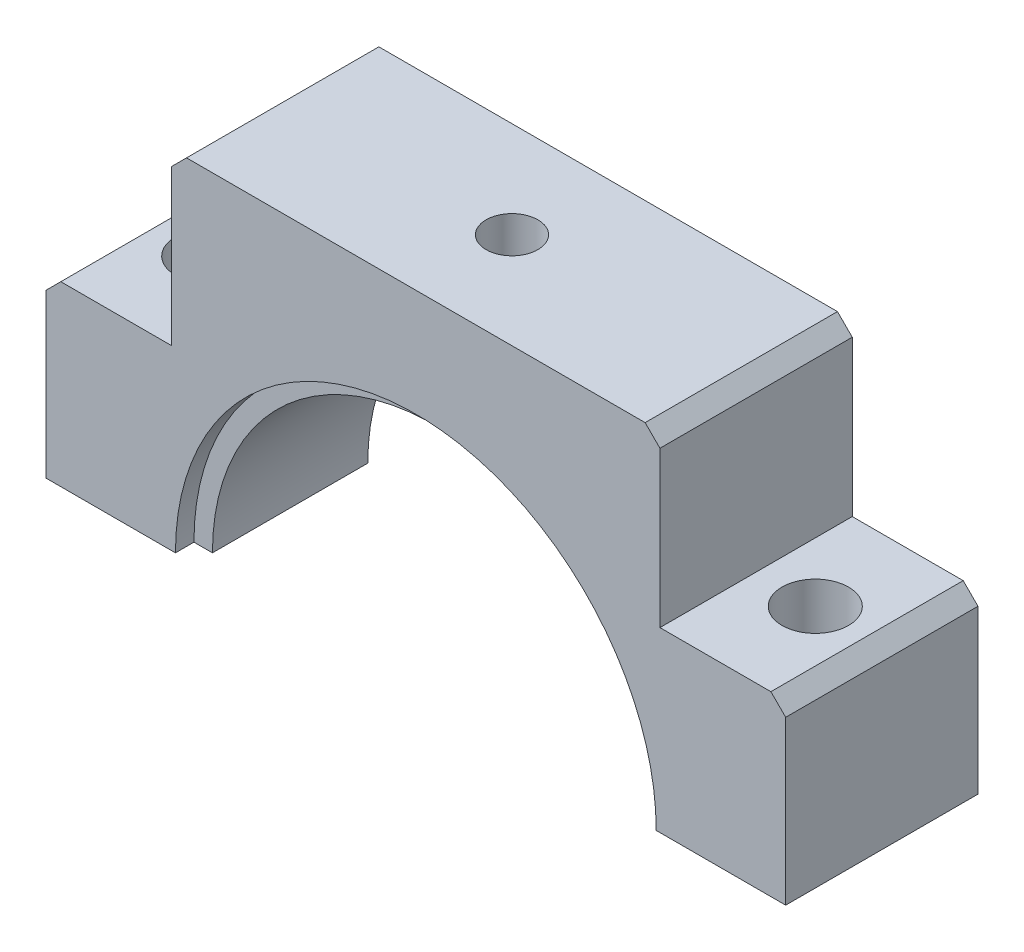
SolidWorks part; units mm, degrees
material "Q235-A"
ref_plane "Front Plane" through (0, 0, 0) normal (0, 0, 1) x (1, 0, 0)
ref_plane "Top Plane" through (0, 0, 0) normal (0, 1, 0) x (1, 0, 0)
ref_plane "Right Plane" through (0, 0, 0) normal (1, 0, 0) x (0, 0, -1)
sketch "Sketch1" plane through (0, 0, 0) normal (0, 0, 1) x (1, 0, 0)
  line L0 (-50, 24) -> (-33, 24)
  line L1 (-50, 0) -> (-30, 0)
  line L2 (-50, 0) -> (-50, 24)
  line L3 (-33, 47) -> (33, 47)
  line L5 (-33, 24) -> (-33, 47)
  line L6 (0, 58.7143) -> (0, -17.0907) construction
  line L7 (50, 0) -> (50, 24)
  line L8 (50, 24) -> (33, 24)
  line L9 (33, 24) -> (33, 47)
  line L10 (30, 0) -> (50, 0)
  arc A0 (30, 0) -> (-30, 0) centre (0, 0) ccw
  point P13 (0, 47)
  dimension "D1" = 100
  dimension "D2" = 47
  dimension "D3" = 23
  dimension "D4" = 33
extrude "Boss-Extrude1" add sketch "Sketch1" along normal blind 26
chamfer "Chamfer1" distance 2 angle 45 4 edges at (50, 24, 13) (33, 47, 13) (-33, 47, 13) (-50, 24, 13)
sketch "Sketch2" plane through (0, 47, 0) normal (0, 1, 0) x (1, 0, 0)
  line L0 (50, -13) -> (-50, -13)
  line L2 (50, 0) -> (50, -26) construction
  line L3 (-50, -26) -> (-50, 0) construction
  line L4 (-41, -7.0808) -> (-41, -18.9192)
  line L5 (41, -7.0808) -> (41, -18.9192)
  point P10 (-41, -13)
  point P11 (41, -13)
  dimension "D1" = 100
  dimension "D2" = 82
  dimension "D3" = 9
hole_wizard "M8x1.0 Tapped Hole1" positions "Sketch3" profile "Sketch4" tap size "M8x1.0" standard "GB"
sketch "Sketch3" plane through (0, 47, 0) normal (0, 1, 0) x (1, 0, 0)
  line L0 (50, -13) -> (-50, -13) construction
  point P0 (0, -13)
sketch "Sketch4" plane through (0, 47, 13) normal (1, 0, 0) x (0, 0, 1)
  line L0 (0, 0) -> (0, 13.103)
  line L1 (0, 13.103) -> (3.5, 11)
  line L2 (3.5, 11) -> (3.5, 0)
  line L5 (3.5, 0) -> (0, 0)
  line L10 (0, 13.103) -> (-3.5, 11) construction
  line L11 (0, -6.35) -> (0, 107.95) construction
  dimension "螺纹孔钻头直径" = 7
  dimension "螺纹孔钻头深度" = 11
  dimension "导头角度" = 118
cosmetic thread "Cosmetic Thread1" parameters "D1"=8, "D2"=8
hole_wizard "Hole2" positions "Sketch9" profile "Sketch10" legacy end condition through all
sketch "Sketch9" plane through (0, 24, 0) normal (0, 1, 0) x (1, 0, 0)
  line L0 (-41, -7.0808) -> (-41, -18.9192) construction
  line L1 (41, -7.0808) -> (41, -18.9192) construction
  point P0 (-41, -13)
  point P4 (41, -13)
sketch "Sketch10" plane through (-41, 24, 13) normal (1, 0, 0) x (0, 0, 1)
  line L0 (0, 0) -> (0, 24)
  line L1 (0, 24) -> (4.5, 24)
  line L2 (4.5, 24) -> (4.5, 0)
  line L3 (4.5, 0) -> (0, 0)
  line L4 (0, 110) -> (0, -10) construction
  dimension "直径" = 9
  dimension "深度" = 24
sketch "Sketch11" plane through (0, 0, 26) normal (0, 0, 1) x (1, 0, 0)
  circle A0 centre (0, 0) radius 32.5
extrude "Cut-Extrude1" cut sketch "Sketch11" against normal blind 2.5
sketch "Sketch12" plane through (0, 0, 0) normal (0, 0, -1) x (-1, 0, 0)
  circle A1 centre (0, 0) radius 32.5
  circle A2 centre (0, 0) radius 32.5
  dimension "D1" = 0
extrude "Cut-Extrude2" cut sketch "Sketch12" against normal blind 2.5
hole_wizard "Hole3" positions "Sketch14" profile "Sketch13" legacy end condition through all
sketch "Sketch14" plane through (0, 47, 0) normal (0, 1, 0) x (1, 0, 0)
  point P0 (0, -13)
sketch "Sketch13" plane through (0, 47, 13) normal (1, 0, 0) x (0, 0, 1)
  line L0 (0, 0) -> (0, 47)
  line L1 (0, 47) -> (2, 47)
  line L2 (2, 47) -> (2, 0)
  line L3 (2, 0) -> (0, 0)
  line L4 (0, 110) -> (0, -10) construction
  dimension "直径" = 4
  dimension "深度" = 47
